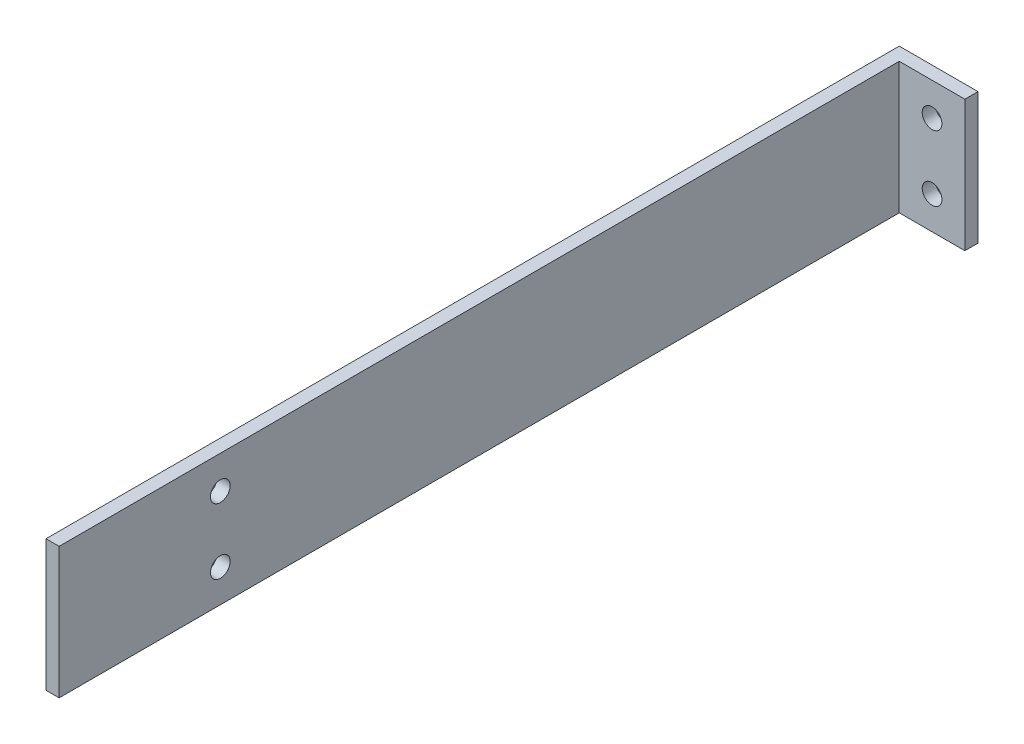
from build123d import *

# Parameters (mm, degrees)
SKETCH1_W           = 2
SKETCH1_H           = 20
BOSS_EXTRUDE1_DEPTH = 130
SKETCH2_W           = 10
SKETCH2_H           = 20
BOSS_EXTRUDE2_DEPTH = 2
SKETCH3_R           = 1.5
CUT_EXTRUDE1_DEPTH  = 6
SKETCH5_R           = 1.5
CUT_EXTRUDE2_DEPTH  = 45


with BuildPart() as part:
    # Sketch1 → Boss-Extrude1 (new body)
    with BuildSketch(Plane.XY):
        with Locations((11, 0)):
            Rectangle(SKETCH1_W, SKETCH1_H)
    extrude(amount=BOSS_EXTRUDE1_DEPTH)

    # Sketch2 → Boss-Extrude2 (add)
    with BuildSketch(Plane.XY):
        with Locations((17, 0)):
            Rectangle(SKETCH2_W, SKETCH2_H)
    extrude(amount=BOSS_EXTRUDE2_DEPTH)

    # Sketch3 → Cut-Extrude1 (cut)
    with BuildSketch(Plane.XY.offset(2)):
        with Locations((17, 5)):
            Circle(SKETCH3_R)
        with Locations((17, -5)):
            Circle(SKETCH3_R)
    extrude(amount=-CUT_EXTRUDE1_DEPTH, mode=Mode.SUBTRACT)

    # Sketch5 → Cut-Extrude2 (cut)
    with BuildSketch(Plane(origin=(12, 0, 0), x_dir=(0, 0, -1), z_dir=(1, 0, 0))):
        with Locations((-105.442155364, -5)):
            Circle(SKETCH5_R)
        with Locations((-105.442155364, 5)):
            Circle(SKETCH5_R)
    extrude(amount=-CUT_EXTRUDE2_DEPTH, mode=Mode.SUBTRACT)


solid = part.part
